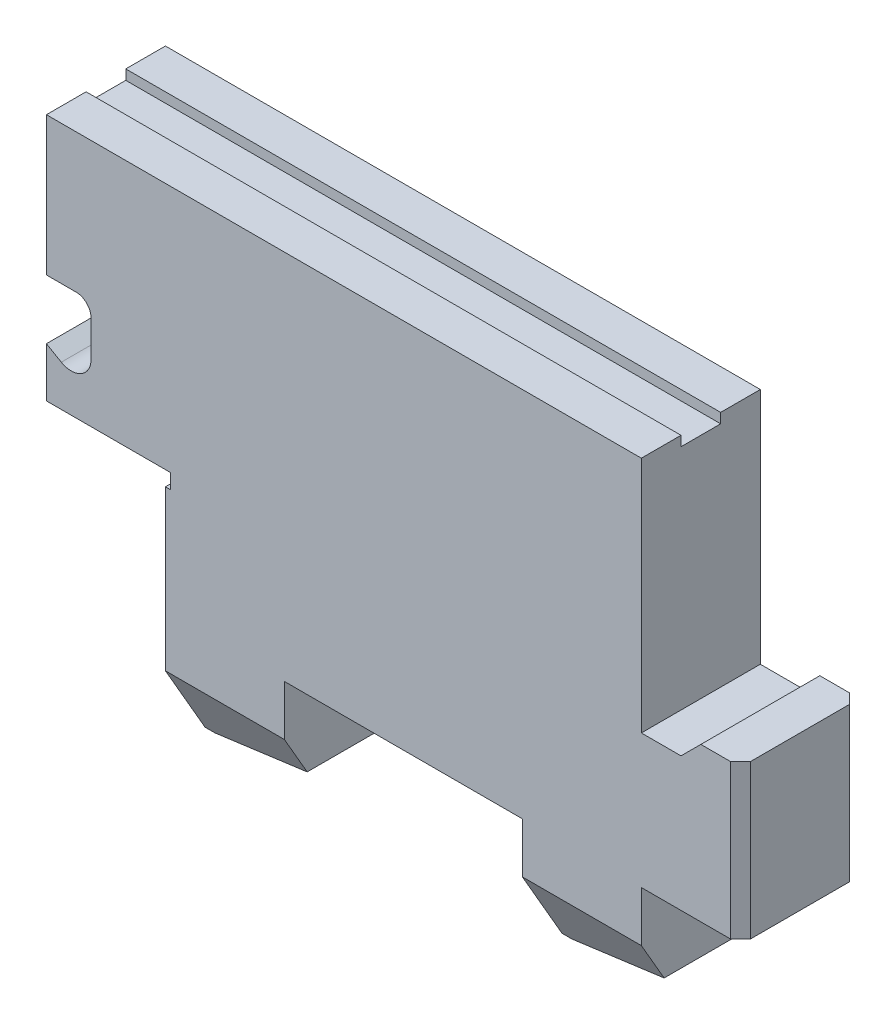
SolidWorks part; units mm, degrees
ref_plane "前视基准面" through (0, 0, 0) normal (0, 0, 1) x (1, 0, 0)
ref_plane "上视基准面" through (0, 0, 0) normal (0, 1, 0) x (1, 0, 0)
ref_plane "右视基准面" through (0, 0, 0) normal (1, 0, 0) x (0, 0, -1)
sketch "草图1" plane through (0, 0, 0) normal (0, 0, 1) x (1, 0, 0)
  line L0 (0, 0) -> (0, 5)
  line L1 (1.5, 4.134) -> (0, 5)
  line L2 (4.5, 5.866) -> (4.5, 9.5)
  line L3 (3, 11) -> (0, 11)
  line L4 (0, 11) -> (0, 25)
  line L5 (0, 25) -> (60, 25)
  line L6 (60, 25) -> (60, 1)
  line L7 (60, 1) -> (64, 1)
  line L8 (64, 1) -> (66, 3)
  line L9 (66, 3) -> (70, 3)
  line L10 (70, 3) -> (70, -12.5)
  line L11 (70, -12.5) -> (60, -12.5)
  line L12 (60, -21.5526) -> (60, -12.5)
  line L13 (60, -21.5526) -> (49, -24.5)
  line L14 (49, -24.5) -> (48, -24.5)
  line L15 (48, -24.5) -> (48, -12.5)
  line L16 (48, -12.5) -> (24, -12.5)
  line L17 (24, -12.5) -> (24, -21.5526)
  line L18 (24, -21.5526) -> (13, -24.5)
  line L19 (13, -24.5) -> (12, -24.5)
  line L20 (12, -1.5) -> (12, -24.5)
  line L22 (12.5, 0) -> (12.5, -1.5)
  line L23 (12.5, 0) -> (0, 0)
  line L24 (12.5, -1.5) -> (12, -1.5)
  arc A0 (1.5, 4.134) -> (4.5, 5.866) centre (2.5, 5.866) ccw
  arc A1 (4.5, 9.5) -> (3, 11) centre (3, 9.5) ccw
  dimension "D13" = 2
  dimension "D15" = 11
  dimension "D1" = 24.5
  dimension "D3" = 1
  dimension "D4" = 4
  dimension "D5" = 45
  dimension "D6" = 2
  dimension "D7" = 15
  dimension "D8" = 15
  dimension "D9" = 1
  dimension "D10" = 12
  dimension "D11" = 10
  dimension "D12" = 12
  dimension "D14" = 60
  dimension "D16" = 3
  dimension "D17" = 12
  dimension "D18" = 49.5
  dimension "D19" = 36
  dimension "D20" = 60
  dimension "D21" = 5
  dimension "D22" = 1.5
  dimension "D23" = 0.5
  dimension "D24" = 4.5
extrude "凸台-拉伸1" add sketch "草图1" along normal mid plane 12
sketch "草图2" plane through (12, 0, 0) normal (-1, 0, 0) x (0, 0, 1)
  line L0 (0, -24.5) -> (0, -16.2947) construction
  line L1 (6, -17.5718) -> (6, -29.5)
  line L2 (2, -24.5) -> (6, -17.5718)
  line L3 (6, -24.5) -> (-6, -24.5) construction
  line L4 (-2, -24.5) -> (2, -24.5)
  line L5 (-2, -24.5) -> (-6, -17.5718)
  line L7 (-6, -1.5) -> (-6, -24.5) construction
  line L8 (-6, -17.5718) -> (-6, -29.5)
  line L9 (-6, -29.5) -> (6, -29.5)
  point P11 (0, -29.5)
  dimension "D1" = 2
  dimension "D2" = 60
  dimension "D3" = 5
extrude "切除-拉伸1" cut sketch "草图2" against normal through all
sketch "草图3" plane through (0, 25, 0) normal (0, 1, 0) x (1, 0, 0)
  line L0 (0, -6) -> (0, 6) construction
  line L1 (0, 2) -> (60, 2)
  line L2 (0, 2) -> (0, -2)
  line L3 (0, -2) -> (60, -2)
  line L4 (60, 2) -> (60, -2)
  line L5 (60, -6) -> (60, 6) construction
  dimension "D1" = 4
  dimension "D2" = 2
extrude "切除-拉伸2" cut sketch "草图3" against normal blind 1
chamfer "倒角1" distance 1 angle 45 2 edges at (70, -4.75, -6) (70, -4.75, 6)
